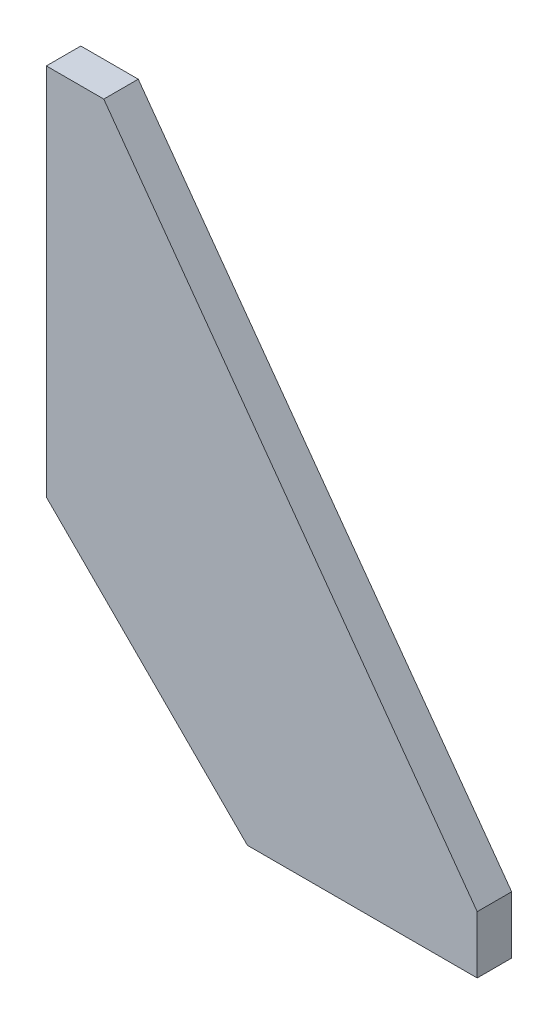
SolidWorks part; units mm, degrees
material "Q235B"
ref_plane "Front Plane" through (0, 0, 0) normal (0, 0, 1) x (1, 0, 0)
ref_plane "Top Plane" through (0, 0, 0) normal (0, 1, 0) x (1, 0, 0)
ref_plane "Right Plane" through (0, 0, 0) normal (1, 0, 0) x (0, 0, -1)
sketch "Sketch1" plane through (0, 0, 0) normal (0, 0, 1) x (1, 0, 0)
  line L0 (0, 100) -> (0, 0)
  line L1 (0, 0) -> (75, 0)
  line L2 (75, 0) -> (75, 10)
  line L3 (75, 10) -> (10, 100)
  line L4 (10, 100) -> (0, 100)
  dimension "D1" = 75
  dimension "D2" = 10
  dimension "D3" = 100
  dimension "D4" = 10
extrude "Boss-Extrude1" add sketch "Sketch1" along normal mid plane 6
chamfer "Chamfer1" distance 35 angle 45 1 edges at (0, 0, 0)
